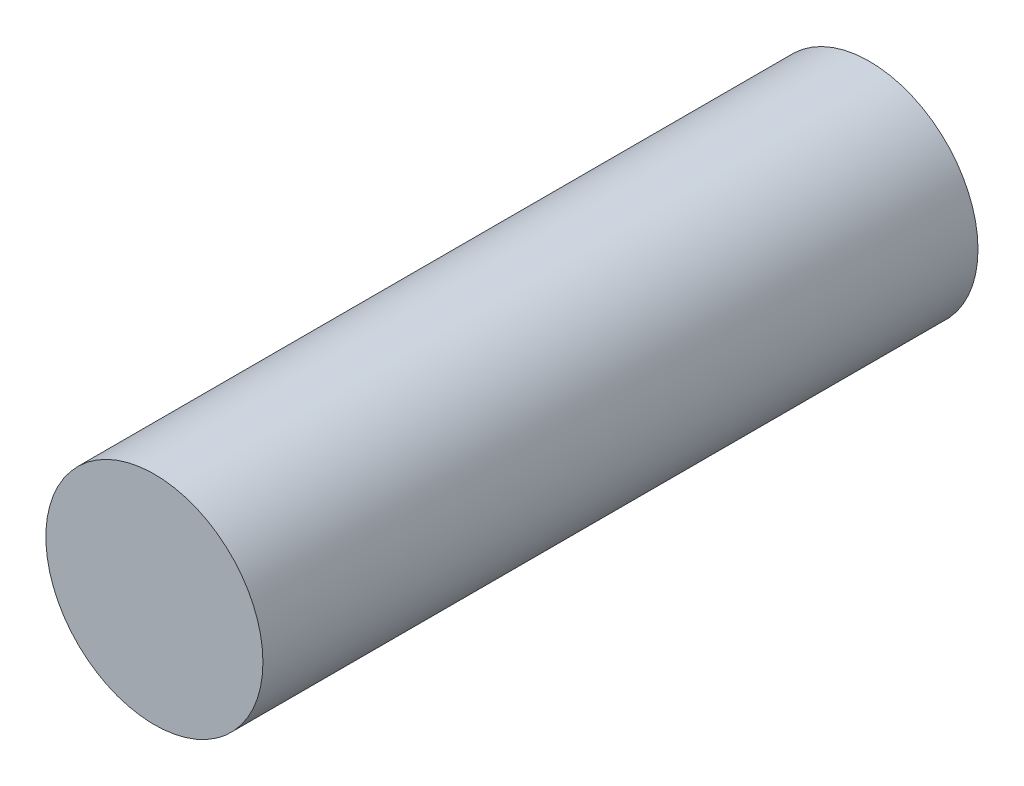
SolidWorks part; units mm, degrees
ref_plane "Front Plane" through (0, 0, 0) normal (0, 0, 1) x (1, 0, 0)
ref_plane "Top Plane" through (0, 0, 0) normal (0, 1, 0) x (1, 0, 0)
ref_plane "Right Plane" through (0, 0, 0) normal (1, 0, 0) x (0, 0, -1)
sketch "Sketch1" plane through (0, 0, 0) normal (0, 0, 1) x (1, 0, 0)
  circle A0 centre (0, 0) radius 40
  dimension "D1" = 80
extrude "Boss-Extrude1" add sketch "Sketch1" along normal blind 263.5
